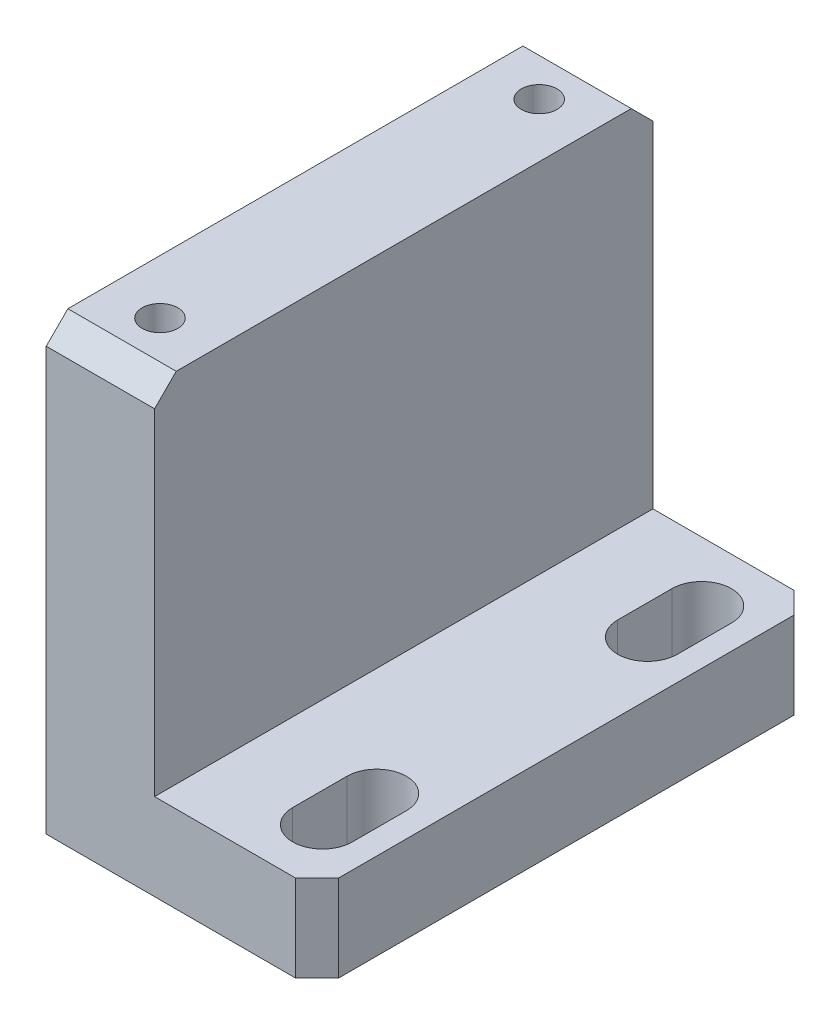
SolidWorks part; units mm, degrees
material "A6061"
ref_plane "Front Plane" through (0, 0, 0) normal (0, 0, 1) x (1, 0, 0)
ref_plane "Top Plane" through (0, 0, 0) normal (0, 1, 0) x (1, 0, 0)
ref_plane "Right Plane" through (0, 0, 0) normal (1, 0, 0) x (0, 0, -1)
sketch "Sketch1" plane through (0, 0, 0) normal (0, 0, 1) x (1, 0, 0)
  line L0 (0, 41) -> (10, 41)
  line L1 (0, 0) -> (25, 0)
  line L2 (0, 0) -> (0, 41)
  line L3 (25, 8) -> (25, 0)
  line L7 (25, 8) -> (10, 8)
  line L8 (10, 41) -> (10, 8)
  dimension "D1" = 10
  dimension "D2" = 8
  dimension "D3" = 25
  dimension "D4" = 41
extrude "Boss-Extrude1" add sketch "Sketch1" along normal mid plane 46
sketch "Sketch2" plane through (0, 0, 0) normal (0, 1, 0) x (1, 0, 0)
  line L0 (20, 17.5) -> (20, 12.5) construction
  line L1 (22.75, 17.5) -> (22.75, 12.5)
  line L2 (17.25, 17.5) -> (17.25, 12.5)
  line L3 (20, -12.5) -> (20, -17.5) construction
  line L4 (22.75, -12.5) -> (22.75, -17.5)
  line L5 (17.25, -12.5) -> (17.25, -17.5)
  line L6 (0, 0) -> (52.3308, 0) construction
  line L9 (25, -23) -> (25, 23) construction
  arc A0 (22.75, 17.5) -> (17.25, 17.5) centre (20, 17.5) ccw
  arc A1 (17.25, 12.5) -> (22.75, 12.5) centre (20, 12.5) ccw
  arc A2 (22.75, -12.5) -> (17.25, -12.5) centre (20, -12.5) ccw
  arc A3 (17.25, -17.5) -> (22.75, -17.5) centre (20, -17.5) ccw
  point P2 (20, 15)
  point P7 (20, -15)
  dimension "D1" = 30
  dimension "D3" = 2.75
  dimension "D4" = 5
  dimension "D2" = 5
extrude "Cut-Extrude1" cut sketch "Sketch2" along normal through all
hole_wizard "M4 Tapped Hole1" positions "Sketch10" profile "Sketch9" tap size "M4" standard "ISO"
sketch "Sketch10" plane through (0, 41, 0) normal (0, 1, 0) x (1, 0, 0)
  line L0 (0, 0) -> (16.8548, 0) construction
  line L1 (5, 23) -> (5, 29.4511) construction
  line L2 (10, 23) -> (0, 23) construction
  point P0 (5, 17.5)
  point P2 (5, -17.5)
  dimension "D1" = 35
sketch "Sketch9" plane through (5, 41, -17.5) normal (1, 0, 0) x (0, 0, 1)
  line L0 (0, 0) -> (0, 11.0914)
  line L1 (0, 11.0914) -> (1.65, 10.1)
  line L2 (1.65, 10.1) -> (1.65, 0)
  line L5 (1.65, 0) -> (0, 0)
  line L10 (0, 11.0914) -> (-1.65, 10.1) construction
  line L11 (0, -6.35) -> (0, 107.95) construction
  dimension "螺纹孔钻头直径" = 3.3
  dimension "螺纹孔钻头深度" = 10.1
  dimension "导头角度" = 118
cosmetic thread "Hole thread3" parameters "D1"=8, "D2"=4
cosmetic thread "Hole thread4" parameters "D1"=8, "D2"=4
chamfer "Chamfer4" distance 2 angle 45 4 edges at (5, 41, 23) (5, 41, -23) (25, 4, 23) (25, 4, -23)
